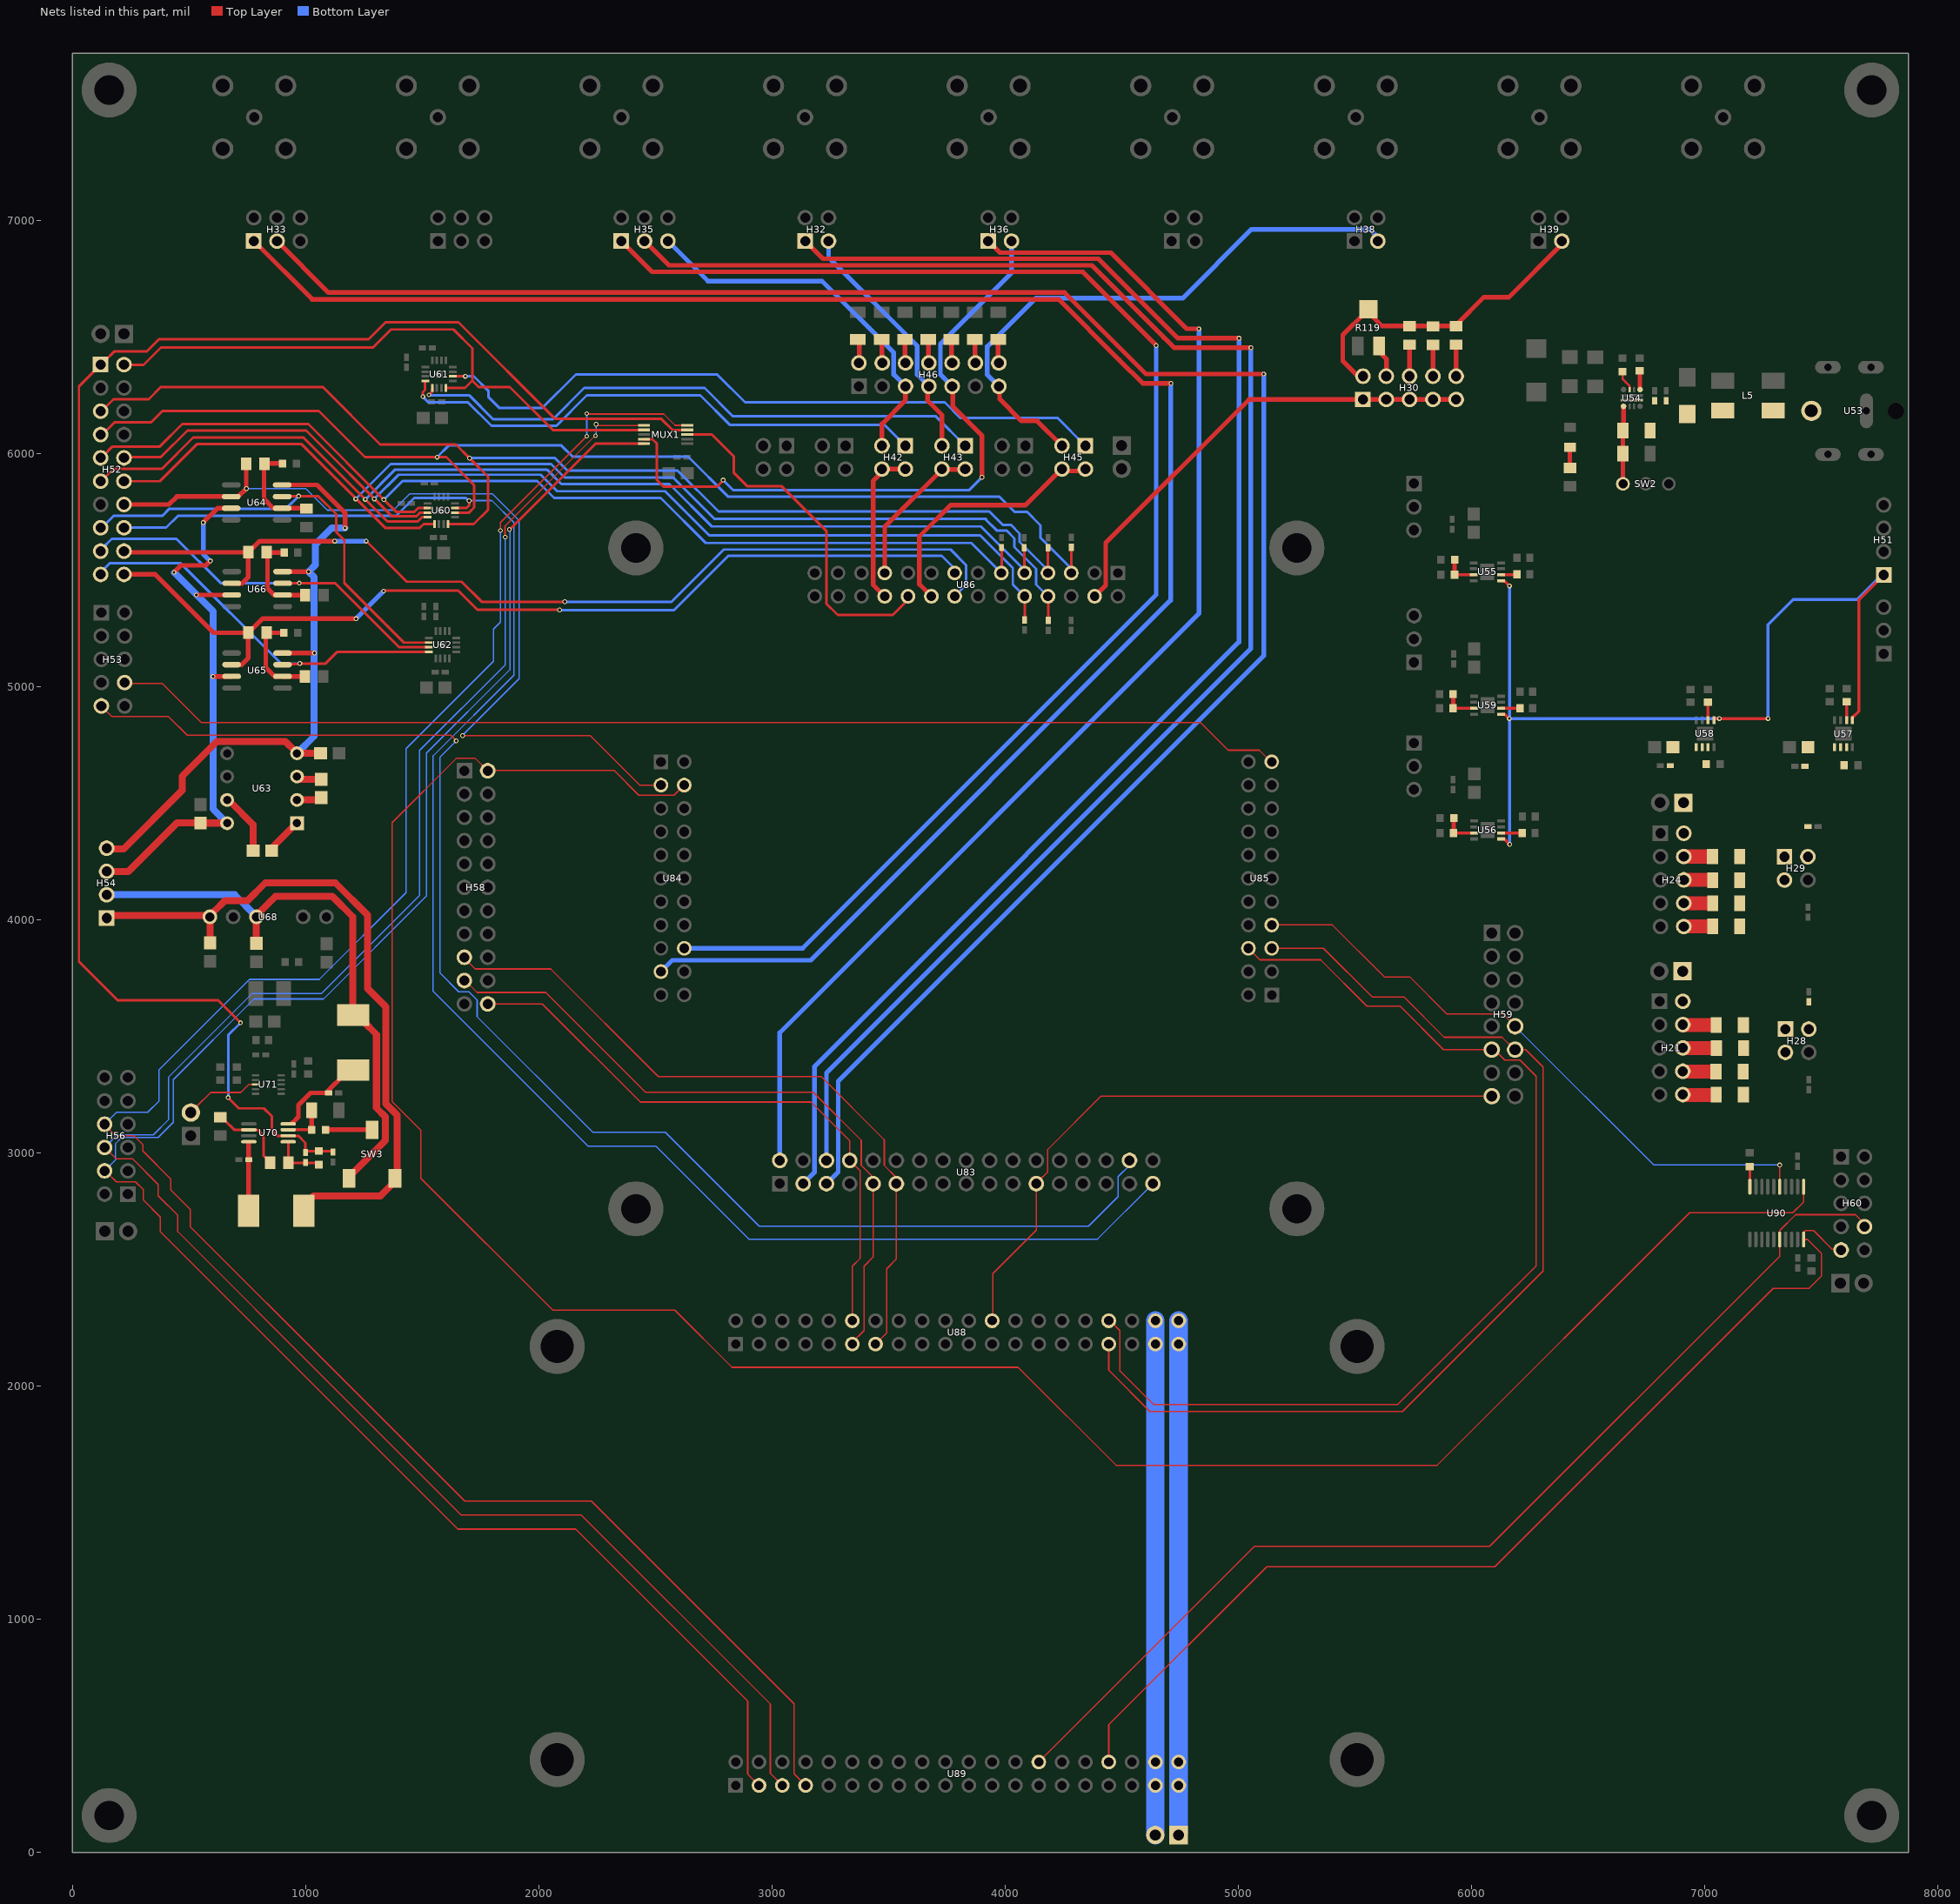
[diagram p0: the nets of this part, all layers, seen from the top]
# Altium PCB MISC62793.pcbdoc (part 4 of 6)
Units mil, origin at the board's own origin, x right, y up, seen from the top; angles counter-clockwise.
Board outline 7874.02 x 7716.54 mil, 4 copper layers (Top Layer, GND, VCC, Bottom Layer); 201 components, 197 nets, 941 pads, 1215 vias.

## Via types
v1: diameter 20, hole 12, Top Layer to Bottom Layer, 1215 vias

## Nets (pads, with @x,y where several pads share a name; then routed paths per layer and width w, separated by ;. In a path a pad name is that pad's centre, name@x,y a point inside that pad or via, vN(x,y) a via of type N, cw(c..) or ccw(c..) an arc to the next point about the centre after c; other vN are vias at no path point) (continued)
EGG: H33.1 U84.19 | length 7962.8
  Top Layer w20: H33.1@777.64,6911 H33.1@781.82,6906.82 ; H33.1@782,6907 1028,6661 4230,6661 4490,6401 4590,6301 v1(4711,6301)
  Bottom Layer w20: U84.19@2523.81,3777.46 2572.35,3826 3166,3826 4710,5370 v1@4710,6301
EGS: H35.1 U84.18 | length 6200.7
  Top Layer w20: H35.1@2353.8,6911 2485.8,6779 4333,6779 v1@4648,6464
  Bottom Layer w20: U84.18@2623.81,3877.46 3131.46,3877.46 4648,5394 v1(4648,6463)
EN_LDO: H51.1 U55.5 U56.5 U57.5 U58.5 U59.5 | length 3980
  Top Layer w13: U55.5@6126.18,5454.08 6140.92,5454.08 v1(6163,5432) ; U56.5@6127.03,4346.59 6140.41,4346.59 v1(6164,4323) ; U59.5@6127.03,4881.59 6143.41,4881.59 v1(6162,4863) ; U58.5@7045,4863 v1(7063,4863) v1(7272,4863) ; U57.5@7634.05,4856.01 7634.05,4867.05 7661,4894 7661,5371 H51.1@7751,5461
  Bottom Layer w13: v1@6163,4323 v1@6163,4863 ; v1(6163,5432) v1@6163,4863 ; v1(7063,4863) v1@6163,4863 ; v1(7272,4863) 7272,5266 7380,5374 7655,5374 H51.1@7743,5462
EN_SL_MUX: H56.4 MUX1.5 U89.3 | length 8609.4
  Top Layer w6: H56.4@150,2914 188,2876 271,2876 304,2843 304,2798 377,2725 377,2662 1086,1953 ; 1073,1966 1086,1953 ; U89.3@2944.4,287 2896,335.4 2896,648 2158,1386 1653,1386 1086,1953
  Top Layer w11: v1(1874,5674) 1876,5674 2243.68,6041.68 MUX1.5@2451.49,6041.68
  Bottom Layer w6: H56.4@138,2923 184,2969 184,3039 210.46,3065.46 367.46,3065.46 433,3131 433,3314 779,3660 1077,3660 1519,4102 1519,4715 1876,5072 v1@1876,5666
  Bottom Layer w11: v1(1874,5674) v1@1876,5672
FPGA_3V3: H57.2 U88.37 U88.38 U89.37 U89.38 | length 2206
  Bottom Layer w80: H57.2@4644,74 4644,387 U88.38@4644,2280
FPGA_5V: H57.1 U88.39 U88.40 U89.39 U89.40 | length 2194.5
  Bottom Layer w80: H57.1@4744.4,85.4 U89.39@4744.4,287 U89.40@4744.4,387 U88.39@4744.4,2179.91 U88.40@4744.4,2279.91
LDO_AVDD: C142.2 C148.2 C151.2 H29.2 R98.2 U58.1 U58.2 U58.3
LDO_DVDD: C139.2 C147.2 C149.2 H28.2 R97.2 U57.1 U57.2 U57.3
MODE: H58.2 U84.4 U90.1 | length 10005.8
  Top Layer w6: H58.2@1779,4647 1785,4641 2322,4641 2429,4534 2580.35,4534 U84.4@2623.81,4577.46 ; H58.2@1781,4639 1728,4692 1646,4692 1371,4417 1371,3220 1494,3097 1494,2891 2060,2325 2584,2325 2829,2080 4056,2080 4476,1660 5853,1660 6936,2743 7378,2743 7424.3,2789.3 U90.1@7424.3,2854.74
MODE_3V3: H60.9 U89.34 U90.20 | length 4419.7
  Top Layer w6: U89.34@4444.4,387 4444.4,547.4 5122,1225 6100,1225 7293.5,2418.5 7447.5,2418.5 7501,2472 7501,2569 7441.32,2628.68 U90.20@7424.3,2628.68 7424.3,2659.3 7432,2667 7467,2667 7548,2586 H60.9@7564,2586
NCSVB: C208.1 H52.7 U60.10 U86.5 | length 5045.8
  Top Layer w11: H52.7@133,6086 180,6133 337,6133 386,6182 1057,6182 1255,5984 v1(1564,5984) 1603,5984 1723,5864 1723,5768 1701.41,5746.41 U60.10@1641.18,5746.41 ; U86.5@4284,5509 C208.1@4284,5597
  Bottom Layer w11: v1(1564,5984) 1614,6034 2097,6034 2145,5986 2641,5986 2813,5814 3976,5814 4040,5750 4094,5750 4152,5692 4152,5638 4283.65,5506.35 U86.5@4283.65,5487.31
NEG_5V: H52.20 R116.2 U65.6 U86.15 | length 4068.1
  Top Layer w11: v1@1340,5411 1656,5411 1738,5329 v1(2089,5329)
  Top Layer w20: H52.20@238,5482 354,5482 604.93,5231.07 R116.2@754.75,5231.07 814.68,5291 v1(1216,5291) ; U65.6@683.02,5093.87 725.87,5093.87 754,5122 R116.2@754,5216
  Bottom Layer w11: v1(2089,5329) 2091,5327 2579,5327 2813,5561 3728,5561 3783.65,5505.35 U86.15@3783.65,5487.31
  Bottom Layer w20: v1(1216,5291) v1(1335,5410)
NEG_5V_DAC: H52.19 U62.4 U65.3 | length 1695.3
  Top Layer w6: U65.3@917,5093 U65.3@928,5093
  Top Layer w11: U65.3@928,5096 v1@975,5096 ; v1@975,5101 980,5101 v1@978,5099 ; U62.4@1528.69,5149.47 1136.47,5149.47 1086,5099 v1@978,5099 ; v1@975,5096 v1@978,5099 ; v1@975,5096 v1(975,5099) v1@978,5099
  Bottom Layer w11: H52.19@122,5491 161,5530 463,5530 894,5099 v1(975,5099)
NetC126_2: C126.2 U54.7 | length 67.2
  Top Layer w20: U54.7@6722,6283 C126.2@6722,6350.21
NetC130_2: C130.2 U55.6 | length 60.5
  Top Layer w13: U55.6@6126.18,5479.68 C130.2@6186.68,5479.68
NetC133_2: C133.2 U59.6 | length 73.2
  Top Layer w13: U59.6@6127.03,4907.19 C133.2@6200.19,4907.19
NetC136_2: C136.2 U56.6 | length 83.2
  Top Layer w13: U56.6@6127.03,4372.19 C136.2@6210.19,4372.19
NetC140_2: C140.2 U57.6 | length 72.5
  Top Layer w13: U57.6@7608.45,4856.01 C140.2@7608.45,4928.55
NetC143_2: C143.2 U58.6 | length 67.4
  Top Layer w13: U58.6@7014.7,4856.28 C143.2@7014.7,4923.7
NetC160_1: C160.1 U63.3 | length 115.9
  Top Layer w30: U63.3@958,4619 974.63,4602.37 C160.1@1067,4602.37
NetC160_2: C160.2 U63.2 | length 93.7
  Top Layer w30: U63.2@963.39,4514.07 C160.2@1057.07,4514.07
NetC161_1: C161.1 U63.7 | length 253.7
  Top Layer w30: U63.7@675,4508 775.63,4407.37 C161.1@775.63,4296
NetC161_2: C161.2 U63.1 | length 142.4
  Top Layer w30: C161.2@854.37,4296 854.37,4307.37 U63.1@947,4400
NetC189_1: C189.1 R128.2 R129.1 U70.1 | length 209.2
  Top Layer w12: U70.1@926.36,3043.64 R129.1@926.36,2957.05 R128.2@1048.95,2957.05
NetC190_1: C190.1 L6.1 U70.8 | length 291.1
  Top Layer w20: L6.1@755.88,2751.05 U70.8@755.88,3042.12
NetC191_2: C191.2 L7.2 U70.4 | length 375.7
  Top Layer w20: U70.4@945,3129 944,3129 969,3154 969,3205.1 1020.9,3257 C191.2@1098.54,3257 1098.54,3268.54 1164,3334 L7.2@1172,3334 ; L7.2@1178.89,3354.89 L7.2@1204,3354.89
NetC198_2: C198.2 C199.2 D5.2 L5.4 R133.1 U54.5
NetH21_4: H21.4 R99.1 | length 122
  Top Layer w60: H21.4@6916,3548 R99.1@7038,3548
NetH21_6: H21.6 R100.1 | length 119
  Top Layer w60: H21.6@6919,3449 R100.1@7038,3449
NetH21_8: H21.8 R101.1 | length 121
  Top Layer w60: H21.8@6916,3348 R101.1@7037,3348
NetH21_10: H21.10 R102.1 | length 122
  Top Layer w60: H21.10@6913,3248 R102.1@7035,3248
NetH24_4: H24.4 R103.1 | length 103
  Top Layer w60: H24.4@6917,4271 R103.1@7020,4271
NetH24_6: H24.6 R104.1 | length 103
  Top Layer w60: H24.6@6920,4172 R104.1@7023,4172
NetH24_8: H24.8 R105.1 | length 103
  Top Layer w60: H24.8@6917,4071 R105.1@7020,4071
NetH24_10: H24.10 R106.1 | length 103
  Top Layer w60: H24.10@6914,3971 R106.1@7017,3971
NetH30_4: H30.4 R119.1 | length 87.3
  Top Layer w20: R119.1@5610,6431 5634.94,6406.06 H30.4@5634.94,6354.06
NetH30_6: H30.6 R117.1 | length 122.6
  Top Layer w20: H30.6@5734,6344 R117.1@5734,6466.63
NetH30_8: H30.8 R118.1 | length 118.8
  Top Layer w20: H30.8@5834.6,6347.4 R118.1@5834.6,6466.23
NetH30_10: H30.10 U67.1 | length 117.6
  Top Layer w20: H30.10@5934,6349 U67.1@5934,6466.63
NetH46_2: H46.2 R120.1 | length 118.3
  Top Layer w20: H46.2@3374,6375 R120.1@3374,6493.3
NetH46_4: H46.4 R121.1 | length 94.2
  Top Layer w20: H46.4@3472,6395 R121.1@3472,6489.24
NetH46_6: H46.6 R122.1 | length 115.3
  Top Layer w20: H46.6@3571,6379 R122.1@3571,6494.3
NetH46_8: H46.8 R123.1 | length 101.3
  Top Layer w20: H46.8@3671,6390 R123.1@3671,6491.3
NetH46_10: H46.10 R124.1 | length 108.3
  Top Layer w20: H46.10@3770,6387 R124.1@3770,6495.3
NetH46_12: H46.12 R125.1 | length 125.2
  Top Layer w20: H46.12@3871,6365 R125.1@3871,6490.24
NetH46_14: H46.14 R126.1 | length 116.8
  Top Layer w20: H46.14@3970,6382 R126.1@3970,6498.78
NetH47_2: H47.2 U71.3 | length 292.4
  Top Layer w6: H47.2@532,3198 593,3259 722,3259 756.02,3293.02 U71.3@785.07,3293.02
NetL5_1: L5.1 U53.1
NetLED2_1: LED2.1 R135.2 | length 80.6
  Top Layer w20: R135.2@6422,5937.37 LED2.1@6422,6018
NetR91_2: R91.2 R92.1 U55.3 | length 132.4
  Top Layer w13: R91.2@5934.32,5479.68 U55.3@6009.98,5479.68
  Top Layer w20: R91.2@5927.45,5479.67 R92.1@5927.45,5536.45
NetR93_2: R93.2 R94.2 U59.3 | length 133.2
  Top Layer w13: R93.2@5930.19,4907.19 U59.3@6010.83,4907.19
  Top Layer w20: R93.2@5921.59,4915.41 R94.2@5921.59,4967.99
NetR95_1: R95.1 R96.2 U56.3 | length 139.6
  Top Layer w13: R96.2@5933.81,4372.19 U56.3@6010.83,4372.19
  Top Layer w20: R96.2@5923.59,4371.99 R95.1@5923.59,4434.59
NetR108_2: R108.2 R111.2 R112.1 U64.2 | length 427.7
  Top Layer w20: R108.2@897,5957 825,5957 822,5954 822,5805 861.93,5765.07 U64.2@899.54,5765.07 R111.2@1007.93,5765.07
NetR109_2: R109.2 R113.2 R114.1 U66.2 | length 391.9
  Top Layer w20: R109.2@907.73,5575.07 836.93,5575.07 836.93,5421.07 866,5392 R113.2@992,5392
NetR110_2: R110.2 R115.2 R116.1 U65.2 | length 381
  Top Layer w20: U65.2@884,5044 867,5044 829.07,5081.93 829.07,5231.07 R116.1@833.49,5231.07 R110.2@907.46,5231.07 ; U65.2@901.32,5043.87 R115.2@984.13,5043.87
NetR129_2: R129.2 R130.1 U70.6 | length 292.5
  Top Layer w12: R130.1@657,3136 694.15,3098.85 U70.6@756.5,3098.85 794.15,3098.85 820,3073 820,2988 R129.2@833,2975
NetR131_1: R131.1 SW3.2 | length 184.3
  Top Layer w20: R131.1@1085.66,3099 SW3.2@1270,3099
NetR131_2: R131.2 R132.2 U70.3 | length 178.6
  Top Layer w13: U70.3@925.48,3098.85 R131.2@1022.85,3098.85
  Top Layer w20: R131.2@1025.78,3100.78 R132.2@1025.78,3182
NetR133_2: R133.2 SW2.3 U54.1 U82.1 | length 315
  Top Layer w20: SW2.3@6649.31,5883.69 U82.1@6649.31,5998.99 R133.2@6649.31,6098.99 ; R133.2@6652,6098.3 U54.1@6652,6198
NetR134_1: R134.1 U54.9 | length 81.7
  Top Layer w10: R134.1@6649,6343 6649,6318 6662,6305 6678.67,6288.33 U54.9@6678.67,6273.62
NetR137_2: R137.2 U90.10 | length 78.2
  Top Layer w12: U90.10@7193.98,2854.74 R137.2@7193.98,2932.98
NG: H33.3 U83.3 | length 8732.6
  Top Layer w20: H33.3@877.64,6911 1098.64,6690 4255,6690 4604,6341 v1(5109,6341)
  Bottom Layer w20: U83.3@3233.65,2867.63 3284.19,2918.16 3284.19,3307.19 5109,5132 5109,6293 ; 5109,6308 5109,6293 ; v1(5109,6341) 5109,6293
NS: H35.3 U83.32 | length 7046.8
  Top Layer w20: H35.3@2453.8,6911 2557.8,6807 4371,6807 4672,6506 ; 4684,6494 4672,6506 ; v1(5054,6454) 4724,6454 4672,6506
  Bottom Layer w20: U83.32@3233.65,2967.63 3233.65,3342.65 5054,5163 v1(5054,6454)
OPA_NEG: C163.2 H54.4 U63.4 U64.4 U65.4 U66.4 | length 2898.4
  Top Layer w20: U64.4@899.54,5865.07 1048.93,5865.07 1169,5745 v1@1169,5681 ; U65.4@901.32,5143.87 v1(1037.87,5143.87) ; U66.4@901.54,5493.07 v1(1012.93,5493.07)
  Top Layer w30: H54.4@154,4303 219,4303 471,4555 471,4616 619.6,4764.6 913.4,4764.6 U63.4@955,4723 ; U63.4@954.73,4722.73 U63.4@963.39,4714.07 ; U63.4@957,4714 C163.2@1064.63,4714
  Bottom Layer w30: U63.4@963.39,4714.07 1037,4787.68 1037,5469 v1@1014.5,5491.5 ; v1(1012.93,5493.07) 1042,5522.14 1042,5610 1112,5680 v1(1169,5680)
OPA_POS: C162.2 H54.3 U63.8 U64.7 U65.7 U66.7 | length 2483.6
  Top Layer w20: v1(436,5490) 466,5520 572,5520 v1(591,5539) ; v1(531.93,5393.07) U66.7@683.24,5393.07 ; v1(561,5704) 622.07,5765.07 U64.7@681.24,5765.07 ; v1(603,5043) 603.87,5043.87 U65.7@683.02,5043.87
  Top Layer w30: H54.3@147,4207 240,4207 449,4416 C162.2@535,4416 ; C162.2@535,4414.63 C162.2@549,4414.63 U63.8@645.37,4414.63
  Bottom Layer w20: v1(561,5704) 561,5569 v1(591,5539)
  Bottom Layer w30: v1@437,5489 603,5323 v1(603,5043) 603,4779 603,4474.46 U63.8@663.39,4414.07
OTA_TEST_OUT: H53.9 U83.19 | length 6215.7
  Top Layer w6: H53.9@140,4901 170,4871 412,4871 492,4791 1623,4791 v1@1647,4767
  Bottom Layer w6: v1(1646,4767) 1576,4697 1576,3772 1657,3691 1700,3691 1736,3655 1736,3584 2232,3088 2543,3088 2946,2685 4358,2685 4485,2812 4485,2898 4533.65,2946.65 U83.19@4533.65,2967.63
OTA_TEST_VB: H52.16 U60.11 U83.17 | length 7597.3
  Top Layer w11: U60.11@1641.18,5766.09 1690.09,5766.09 1703,5779 v1@1703,5795
  Bottom Layer w6: v1@1703,5798 1799,5798 1893,5704 1893,5049 1547,4703 1547,3693 2212,3028 2503,3028 2901,2630 4396.03,2630 U83.17@4633.65,2867.63
  Bottom Layer w11: H52.16@244,5682 402,5682 453,5733 1389,5733 1465.5,5809.5 1687.5,5809.5 v1@1694,5803
  other v1: 1701,5797
PG: H32.1 U83.2 | length 6463.5
  Top Layer w20: H32.1@3142.61,6911 3218.61,6835 4400,6835 4708,6527 ; 4729,6506 4708,6527 ; v1(5003,6494) 4741,6494 4708,6527
  Bottom Layer w20: U83.2@3133.65,2867.63 3183.12,2917.09 3183.12,3371.12 5003,5191 5003,6320 v1(5003,6494)
PS: H36.1 U83.34 | length 5371.2
  Top Layer w20: H36.1@3927.41,6911 3977.41,6861 4453,6861 4779,6535 v1(4831,6535)
  Bottom Layer w20: U83.34@3033.65,2967.63 3033.65,3515.65 4831,5313 v1(4831,6535)
REG_R_EN: H59.11 U85.6 U88.34 | length 4603.5
  Top Layer w6: U88.34@4460,2270 4492,2238 4492,2065 4637,1920 5038,1920 ; 5019,1920 5038,1920 ; U85.6@5043.5,3877.46 5092.96,3828 5353,3828 5552,3629 5694,3629 5880,3443 H59.11@6087,3443 6098,3443 6143,3398 6208,3398 6277,3329 6277,2515 5682,1920 5038,1920
REG_STATE: H59.10 U85.7 U90.5 | length 2685.4
  Top Layer w6: U85.7@5143.5,3977.46 5403.54,3977.46 5626,3755 5735,3755 5894,3596 6135,3596 H59.10@6179,3552 ; U90.5@7321.93,2854.74 v1(7321.93,2947.93)
  Bottom Layer w6: H59.10@6187,3543 6781,2949 7320,2949 v1@7321,2950
REG_STATE_3V3: H60.8 U89.28 U90.16 | length 4581.6
  Top Layer w6: U89.28@4144.4,387 5069.4,1312 6078,1312 7321.93,2555.93 U90.16@7321.93,2628.68 7321.93,2666.93 7390,2735 7646,2735 H60.8@7676,2705
REG_W_EN: H59.12 U85.5 U88.33 | length 4550.9
  Top Layer w6: U88.33@4444.4,2179.91 4444.4,2067.6 4447,2065 4450,2062 4621,1891 5033,1891 ; 5019,1891 5033,1891 ; U85.5@5143.5,3877.46 5365.54,3877.46 5575,3668 5711,3668 5883,3496 6131,3496 H59.12@6179,3448 ; H59.12@6187,3443 6232,3443 6307,3368 6307,2493 5705,1891 5033,1891
ROW_D_EN: H58.22 U83.31 U88.12 | length 2607.1
  Top Layer w6: H58.22@1781,3639 2015,3639 2436,3218 3168,3218 3333.65,3052.35 U83.31@3333.65,2967.63 3379,2922.28 3379,2548 3344.4,2513.4 U88.12@3344.4,2279.91 ; U88.12@3347,2274 U88.12@3347,2279.91
ROW_L_EN: H58.17 U83.6 U88.13 | length 3038.3
  Top Layer w6: H58.17@1695,3821 1727,3789 2051,3789 2513,3327 3211,3327 3482,3056 3482,2946 3533.65,2894.35 U83.6@3533.65,2867.63 3533.65,2544.65 3492,2503 3492,2227.51 U88.13@3444.4,2179.91
RST_N: H58.19 U83.5 U88.11 | length 2889.9
  Top Layer w6: H58.19@1697,3727 1736,3688 2030,3688 2458,3260 3177,3260 3383,3054 3383,2947 3433.65,2896.35 U83.5@3433.65,2867.63 3433.65,2552.65 3395,2514 3395,2238 U88.11@3344,2187
SAMPLE: H59.15 U83.12 U88.24 | length 2908.1
  Top Layer w6: U88.24@3947,2286 3947,2429 ; 3947,2328 3947,2429 ; U83.12@4133.65,2867.63 4133.65,2668.65 3947,2482 3947,2429 ; U83.12@4145,2881 4183,2919 4183,3015 4411,3243 H59.15@6087,3243
SL_SEL0: H56.6 MUX1.1 U89.5 | length 8734.8
  Top Layer w6: H56.6@152,3010 188,2974 259,2974 368,2865 368,2816 452,2732 452,2662 1116.5,1997.5 ; 1112,2002 1116.5,1997.5 ; v1(1856,5641) 1855,5642 1855,5689 2238,6072 v1@2248,6072 ; v1(2246,6125) 2250.58,6120.42 MUX1.1@2451.49,6120.42 ; U89.5@3044.4,287 2993,338.4 2993,636 2182,1447 1667,1447 1116.5,1997.5
  Bottom Layer w6: H56.6@138,3023 192.46,3077.46 347.46,3077.46 413,3143 413,3326 771,3684 1069,3684 1489,4104 1489,4726 1856,5093 v1(1856,5641) v1@1855,5642 ; v1(2243,6076) 2243,6074 2246,6071 v1(2246,6125)
SL_SEL1: H56.8 MUX1.10 U89.7 | length 9044.5
  Top Layer w6: H56.8@151,3108 186,3073 264,3073 302,3035 302,3008 422,2888 422,2841 505,2758 505,2684 1158,2031 ; 1153,2036 1158,2031 ; v1(1836,5669) 1836,5704 v1@2203,6071 ; v1@2201,6175 2207,6169 2536,6169 2584.57,6120.43 MUX1.10@2636.53,6120.43 ; U89.7@3144.4,287 3095,336.4 3095,637 2226,1506 1683,1506 1158,2031
  Bottom Layer w6: H56.8@138,3123 189,3174 323,3174 371,3222 371,3356 759,3744 1059,3744 1431,4116 1431,4734 1806,5109 1806,5247 1836,5277 v1(1836,5669) ; v1(2206,6074) v1(2206,6171)
SL_TEST: H53.8 U85.21 | length 5056.4
  Top Layer w6: H53.8@226,5014 385,5014 553,4846 4838,4846 4957,4727 5090,4727 U85.21@5142,4675
TIA_+5V: C187.1 H54.1 L6.2 SW3.3 U68.6 | length 2975.3
  Top Layer w30: H54.1@163,4019 248,4019 ; 224.48,4019 248,4019 ; C187.1@590,3900.37 590,4019 248,4019 ; 610,4038 654,4082 751,4082 828,4159 1127,4159 1266,4020 1266,3705 1344,3627 1344,3210 1392,3162 1392,2912 1383.43,2903.43 SW3.3@1383.43,2890.67 ; L6.2@992.1,2751.05 992.1,2773.1 1034,2815 1321,2815 SW3.3@1384,2878
TIA_-5V: C186.1 H54.2 L7.1 SW3.1 U68.4 | length 2448.5
  Top Layer w30: U68.4@784.01,4018.01 U68.4@789.53,4012.48 ; C186.1@789,3898.37 U68.4@789,4002 ; U68.4@802,4031 871,4100 1115,4100 1203,4012 L7.1@1203,3615 ; SW3.1@1186.57,2890.67 1186.57,2897.57 1342,3053 1342,3155 1304,3193 1304,3508 L7.1@1249,3563 ; L7.1@1204,3591.11 L7.1@1204,3615
  Bottom Layer w30: H54.2@147,4107 696,4107 U68.4@785,4018
TP_AVDD: H23.1 H24.2 H29.1 H29.3 R103.2 R104.2 R105.2 R106.2
TP_DVDD: H21.2 H22.1 H28.1 H28.3 R99.2 R100.2 R101.2 R102.2
V_ADC_TEST: H30.1 H30.3 H30.5 H30.7 H30.9 U86.4 | length 2013
  Top Layer w20: U86.4@4383.65,5387.31 4431.15,5434.8 4431.15,5616.15 5046,6231 5834.6,6231 H30.9@5941,6231
V_ADC_TEST_BNC: H30.2 H39.3 R117.2 R118.2 R119.2 U67.2 | length 1362.4
  Top Layer w20: H30.2@5530,6331 5513,6331 5448,6396 5448,6508 5544.74,6604.74 R119.2@5562,6604.74 ; R119.2@5564,6599 5616,6547 U67.2@5938,6547 ; U67.2@5938,6555 6053,6670 6160,6670 6385,6895 H39.3@6385,6899
VB_CLAMP: C202.1 H52.9 U60.2 U86.11 | length 4533.1
  Top Layer w11: H52.9@134,5992 172,6030 375,6030 471,6126 1012,6126 v1(1336,5802) 1388,5750 1467,5750 1483.09,5766.09 U60.2@1523.07,5766.09 ; U86.11@3983,5506 3985,5508 C202.1@3985,5587
  Bottom Layer w11: v1(1336,5802) 1416,5882 1993,5882 2066,5809 2523,5809 2716,5616 3854.96,5616 U86.11@3983.65,5487.31
VB_CM: C204.1 H52.11 U60.4 U86.9 | length 4778.9
  Top Layer w11: H52.11@135,5893 176,5934 384,5934 518,6068 991,6068 v1(1256,5803) 1351,5708 1481,5708 1499.72,5726.72 U60.4@1523.07,5726.72 ; U86.9@4082,5500 C204.1@4082,5590
  Bottom Layer w11: v1(1256,5803) 1384,5931 2035,5931 2097,5869 2560,5869 2742,5687 3896,5687 4083.65,5499.35 U86.9@4083.65,5487.31
VB_CMP: C206.1 H52.5 U60.8 U86.7 | length 4988.6
  Top Layer w11: H52.5@129,6186 176,6233 327,6233 378,6284 1075,6284 1320,6039 1644,6039 v1(1703,5980) 1782,5901 1782,5758 1721.2,5697.2 U60.8@1611.65,5697.2 ; U86.7@4184,5510 C206.1@4184,5595
  Bottom Layer w11: v1(1703,5980) 2070,5980 2123,5927 2595,5927 2771,5751 3932,5751 3989,5694 4025,5694 4062.5,5656.5 4062.5,5620.5 4183.65,5499.35 U86.7@4183.65,5487.31
VBL1: H42.2 H42.4 U86.22 | length 672.4
  Top Layer w20: U86.22@3483.65,5387.31 3434,5436.96 3434,5882 3485,5933 H42.2@3570,5933
VBL1_BNC: H35.5 H42.3 H46.5 | length 1626.2
  Top Layer w20: H42.3@3472,6033 3472,6127 3572,6227 H46.5@3572,6286
  Bottom Layer w20: H35.5@2553.8,6911 2725.8,6739 3215,6739 3522.46,6431.54 3522.46,6338.54 H46.5@3573,6288
VBL1_DAC: H42.1 U61.4 | length 2332
  Top Layer w11: v1(1503,6244) 1503,6263 1512,6272 U61.4@1512,6307
  Bottom Layer w11: v1@1503,6241 1503,6243 1502,6244 v1(1503,6244) ; v1@1505,6241 1526,6220 1696,6220 1797,6119 2076,6119 2206,6249 2693,6249 2819,6123 3482,6123 H42.1@3572,6033
VBL2: H43.2 H43.4 U86.21 | length 635.3
  Top Layer w20: U86.21@3483.65,5487.31 3483.65,5685.65 3729,5931 H43.2@3819,5931
VBL2_BNC: H32.3 H43.3 H46.7 | length 1085.9
  Top Layer w20: H46.7@3668,6285 3668,6226 3729,6165 H43.3@3729,6033
  Bottom Layer w20: H32.3@3242.61,6911 H32.3@3243,6910.61 ; H32.3@3243,6918 H32.3@3243,6910.61 ; H46.7@3673,6288 3623,6338 3623,6461 3243,6841 H32.3@3243,6910.61
VBL2_DAC: H43.1 U61.5 | length 2537.1
  Top Layer w11: v1(1529,6251) 1543.17,6265.17 U61.5@1543.17,6281.39
  Bottom Layer w11: v1@1529,6250 1701,6250 1804,6147 2061,6147 2195,6281 2711,6281 2833,6159 3703,6159 H43.1@3829,6033
VBL_DARK: H45.2 H45.4 U86.18 | length 1103.5
  Top Layer w20: U86.18@3683.65,5387.31 3632,5438.96 3632,5644 3766,5778 4086,5778 4233,5925 H45.2@4341,5925
VBL_DARK_BNC: H38.3 H45.3 H46.13 | length 2499.6
  Top Layer w20: H46.13@3976,6290 3976,6234 4070,6140 4137,6140 H45.3@4244,6033
  Bottom Layer w20: H46.13@3973,6288 3923.54,6337.46 3923.54,6458.54 4131,6666 4761,6666 5056.54,6961.54 5563.46,6961.54 H38.3@5601,6924
VBL_DARK_DAC: H45.1 U61.10 | length 2966.8
  Top Layer w11: U61.10@1631.75,6330.6 v1@1682.4,6330.6
  Bottom Layer w11: v1(1685,6331) 1721,6331 1785,6267 1785,6241 1830,6196 2016,6196 2159,6339 2765,6339 2885,6219 3109,6219 3482,6219 3741,6219 3807,6153 4224,6153 H45.1@4344,6033
VCB: C205.1 H52.12 U60.5 U86.8 | length 4947.7
  Top Layer w11: H52.12@239,5881 375,5881 535,6041 981,6041 1341,5681 1490,5681 1506.2,5697.2 U60.5@1552.6,5697.2 ; C205.1@4185,5283.46 U86.8@4185,5364
  Bottom Layer w11: v1(1215,5805) 1365,5955 2053,5955 2111,5897 2576,5897 2754,5719 3915,5719 ; 3919,5719 3915,5719 ; U86.8@4183.65,5387.31 4133,5437.96 4133,5505 4040,5598 4040,5636 4006,5670 3964,5670 3915,5719
VCLAMP: C203.1 H52.10 U60.3 U86.10 | length 4659.5
  Top Layer w11: H52.10@245,5984 379,5984 493,6098 1003,6098 1371,5730 1475,5730 1491.41,5746.41 U60.3@1523.07,5746.41 ; C203.1@4084,5285.46 U86.10@4084,5371
  Bottom Layer w11: v1(1295,5805) 1399,5909 2008,5909 2079,5838 2542,5838 2731,5649 3893,5649 4033,5509 4033,5437.96 U86.10@4083.65,5387.31
VMH: H52.14 R112.2 U64.6 U84.3 | length 3868
  Top Layer w6: v1@1674,4788 v1@1676,4790 ; v1@1675,4790 v1@1676,4790 ; U84.3@2523.81,4577.46 2433.54,4577.46 2221,4790 v1@1676,4790
  Top Layer w20: H52.14@230,5781 414,5781 448.07,5815.07 U64.6@681.24,5815.07 ; U64.6@710,5814 745.02,5849.02 R112.2@745.02,5956.07
  Bottom Layer w6: v1(745.98,5849.02) 1000.98,5849.02 1093,5757 1377,5757 1447,5827 1801,5827 1916,5712 1916,5034 v1@1673,4791
  other v1: 1673,4790
VMH_DAC: H52.15 U62.2 U64.3 | length 1902.4
  Top Layer w11: U64.3@928,5817 v1(970,5817) 1054,5817 1131,5740 1131,5663 1166,5628 1166,5444 1421.16,5188.84 U62.2@1528.69,5188.84
  Bottom Layer w11: H52.15@134,5690 176,5732 385,5732 416,5763 916,5763 v1(970,5817)
VML: H52.18 R114.2 U66.6 U86.16 | length 4319.9
  Top Layer w11: v1(1260,5624) 1434,5450 1669,5450 1755,5364 1850,5364 ; 1838,5364 1850,5364 ; v1(2112,5364) 1850,5364
  Top Layer w20: H52.18@232.93,5576.07 306,5576.07 ; 274.93,5576.07 306,5576.07 ; 434.93,5576.07 538,5576.07 ; U66.6@683.24,5443.07 728.07,5443.07 754,5469 R114.2@754,5557 ; v1(1125,5624) 802.95,5624 R114.2@755.02,5576.07 538,5576.07 ; 306,5576.07 538,5576.07
  Bottom Layer w11: v1@2110,5364 v1(2112,5364) 2570,5364 2794,5588 3766,5588 3833,5521 3833,5436.65 U86.16@3783.65,5387.31
  Bottom Layer w20: v1(1125,5624) v1(1260,5624)
VML_DAC: H52.17 U62.3 U66.3 | length 1655.8
  Top Layer w11: U66.3@926,5444 v1(973,5444) 1126,5444 1400.84,5169.16 U62.3@1528.69,5169.16
  Bottom Layer w11: H52.17@129,5594 169,5634 446,5634 636,5444 v1(973,5444)
VSL: MUX1.8 U86.20 | length 1513.5
  Top Layer w11: MUX1.8@2636.53,6081.05 2741.95,6081.05 2837,5986 2837,5916 2893,5860 3041,5860 3233,5668 3233,5356 3282,5307 3518,5307 U86.20@3580,5369
VSL_BNC: H36.3 H46.9 MUX1.4 | length 2897.6
  Top Layer w11: MUX1.4@2451.49,6061.37 2487.63,6061.37 2507,6042 2507,5886 2535,5858 2765,5858 2779.5,5872.5 v1@2790,5883
  Top Layer w20: H46.9@3775,6297 3775,6202 3901,6076 v1(3901,5898)
  Bottom Layer w11: v1(2791,5886) 2835,5842 3845,5842 v1(3901,5898)
  Bottom Layer w20: H46.9@3773,6288 3722.46,6338.54 3722.46,6469.46 4028,6775 H36.3@4028,6906 ; H36.3@4027.41,6907 H36.3@4027.41,6911 ; H36.3@4029,6906 H36.3@4029,6907
VSL_DAC: H52.2 MUX1.2 U61.8 | length 2662.4
  Top Layer w11: H52.2@239,6380 305,6380 380,6455 1289,6455 1366,6532 1634,6532 1715,6451 1715,6313 1683.39,6281.39 U61.8@1602.22,6281.39 ; U61.8@1605,6282 U61.8@1607,6282 ; 1715,6312 1742,6285 1876,6285 2060.26,6100.74 MUX1.2@2451.49,6100.74
VSL_TIA: C188.1 C189.2 H52.1 MUX1.9 R128.1 U70.2 | length 7100.1
  Top Layer w11: H52.1@121,6381 28,6288 28,3821 195,3654 626,3654 v1@722,3558 ; H52.1@139,6397 179,6437 318,6437 371,6490 1270,6490 1343,6563 1656,6563 2071,6148 2526,6148 2573.26,6100.74 MUX1.9@2636.53,6100.74 ; v1(668,3237) 714,3191 821,3191 855,3157 855,3098 879.74,3073.26 U70.2@925.48,3073.26 968.74,3073.26 999,3043 999,3007 C188.1@1115,3007
  Bottom Layer w11: v1(668,3237) 668,3505 v1(721,3558)